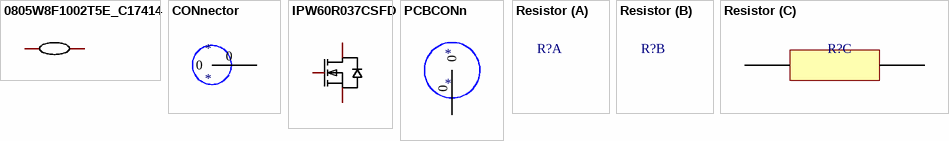
[diagram p0: symbols 0805W8F1002T5E_C17414 to Resistor]
# Altium schematic symbol library MISC82254-8.SchLib: 5 symbols
Pins are listed as number, name and electrical type; pins without a type are passive.


## 0805W8F1002T5E_C17414
designator R?
Tolerance: ±1%
footprint R0805
pins: 1, 2

## CONnector
designator *
footprint CONN-TH_T44001
pins: 0

## IPW60R037CSFD
designator Q?
footprint TO-247-3_L15.9-W5.1-P5.44-L
pins: 1 G, 2 D, 3 S

## PCBCONn
designator *
footprint CONN-TH_T44001
pins: 0

## Resistor
designator R?
Resistor
footprint R_test
part C pins: 0, 1